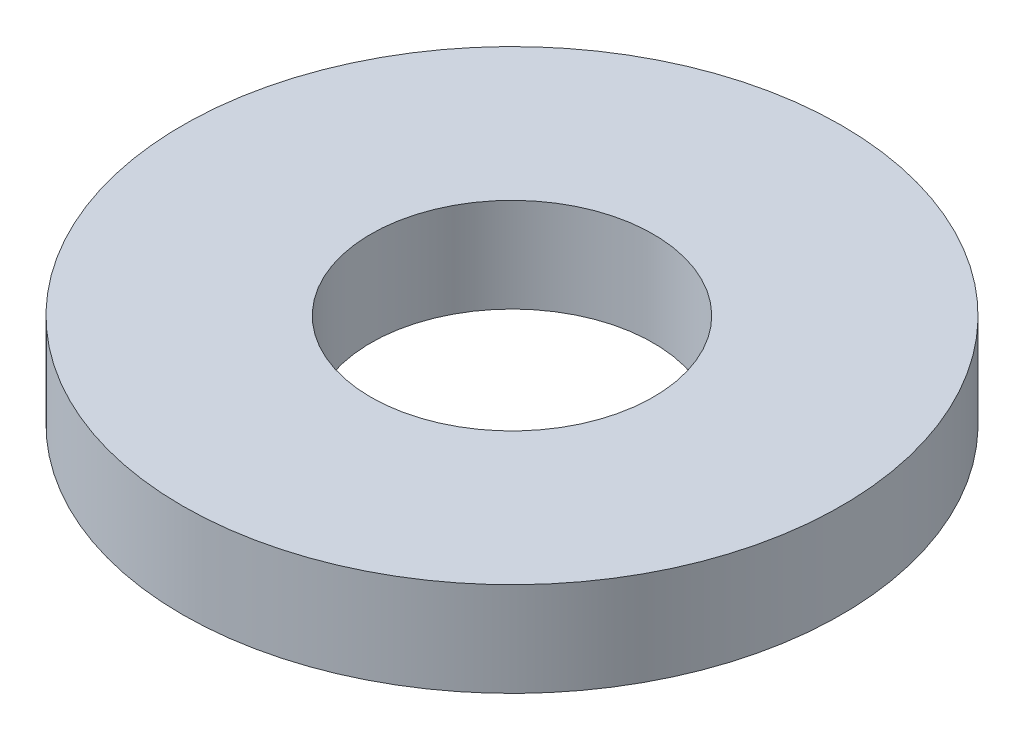
from build123d import *

# Parameters (mm, degrees)
SKETCH1_R           = 5.25
SKETCH1_R_2         = 2.25
BOSS_EXTRUDE1_DEPTH = 1.5


with BuildPart() as part:
    # Sketch1 → Boss-Extrude1 (new body)
    with BuildSketch(Plane(origin=(0, 0, 0), x_dir=(1, 0, 0), z_dir=(0, 1, 0))):
        with Locations(Location((0, 0, 0), (0, 0, 270))):
            Circle(SKETCH1_R)
        with Locations(Location((0, 0, 0), (0, 0, 270))):
            Circle(SKETCH1_R_2, mode=Mode.SUBTRACT)
    extrude(amount=BOSS_EXTRUDE1_DEPTH)


solid = part.part
